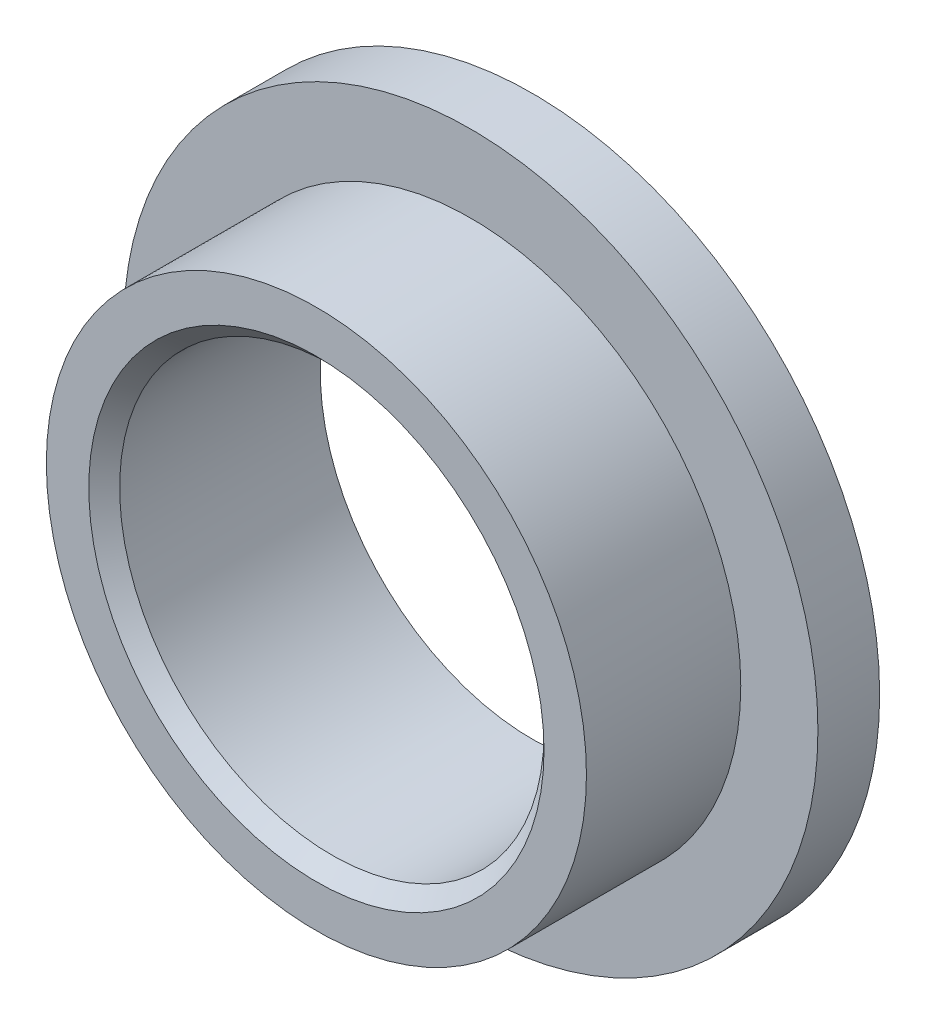
from build123d import *

# Parameters (mm, degrees)
SKETCH1_R           = 45
SKETCH1_R_2         = 27.5
BOSS_EXTRUDE1_DEPTH = 28
CUT_EXTRUDE1_START  = -20
SKETCH2_R           = 45
SKETCH2_R_2         = 35
CUT_EXTRUDE1_DEPTH  = 20
CHAMFER1_SIZE       = 2


with BuildPart() as part:
    # Sketch1 → Boss-Extrude1 (new body)
    with BuildSketch(Plane.XY):
        Circle(SKETCH1_R)
        Circle(SKETCH1_R_2, mode=Mode.SUBTRACT)
    extrude(amount=BOSS_EXTRUDE1_DEPTH)

    # Sketch2 → Cut-Extrude1 (cut)
    with BuildSketch(Plane.XY.offset(28).offset(CUT_EXTRUDE1_START)):
        Circle(SKETCH2_R)
        Circle(SKETCH2_R_2, mode=Mode.SUBTRACT)
    extrude(amount=CUT_EXTRUDE1_DEPTH, mode=Mode.SUBTRACT)

    # Chamfer1
    chamfer1_edges = [part.edges().sort_by_distance(p)[0] for p in [
        (-27.5, 0, 28),
    ]]
    chamfer(chamfer1_edges, length=CHAMFER1_SIZE)


solid = part.part
